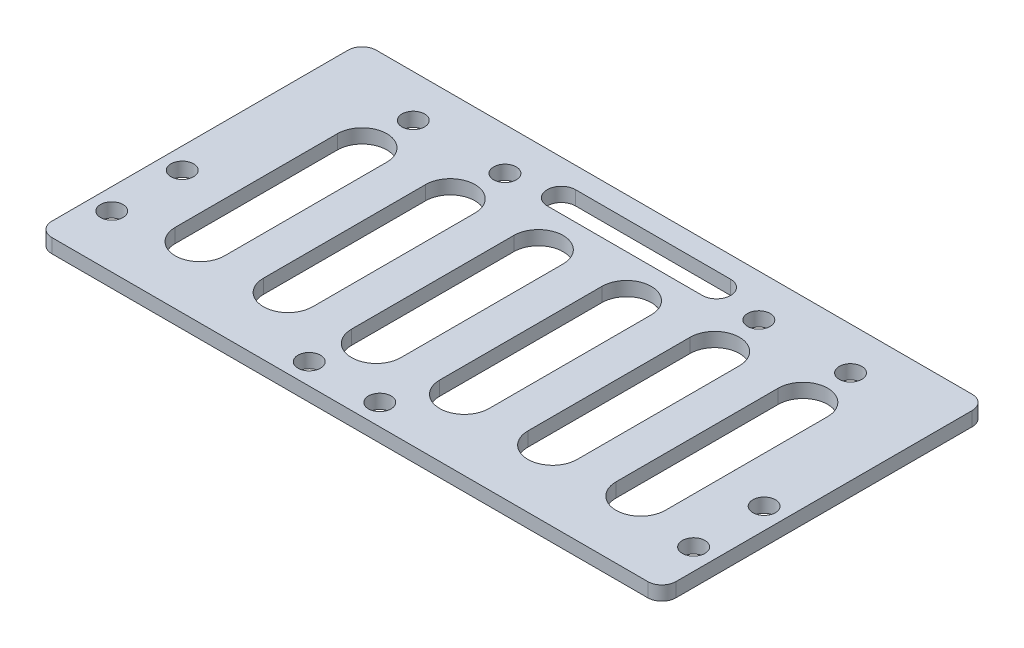
SolidWorks part; units mm, degrees
material "Thornel Mat VMA"
ref_plane "前视基准面" through (0, 0, 0) normal (0, 0, 1) x (1, 0, 0)
ref_plane "上视基准面" through (0, 0, 0) normal (0, 1, 0) x (1, 0, 0)
ref_plane "右视基准面" through (0, 0, 0) normal (1, 0, 0) x (0, 0, -1)
sketch "草图1" plane through (0, 0, 0) normal (0, 1, 0) x (1, 0, 0)
  line L0 (0, 23) -> (0, -23) construction
  line L1 (-44.25, 23) -> (44.25, 23)
  line L2 (-44.25, 23) -> (-44.25, -23)
  line L3 (-44.25, -23) -> (44.25, -23)
  line L4 (44.25, 23) -> (44.25, -23)
  line L5 (-44.25, 23) -> (44.25, -23) construction
  line L6 (-44.25, -23) -> (44.25, 23) construction
  line L7 (-41.25, -5.5) -> (-41.25, -15.5) construction
  line L8 (41.25, -5.5) -> (41.25, -15.5) construction
  line L9 (-8.75, -20) -> (1.25, -20) construction
  line L10 (-31, 17) -> (-18, 17) construction
  line L11 (18, 17) -> (31, 17) construction
  line L12 (-44.25, 0) -> (44.25, 0) construction
  line L13 (-8.75, 20) -> (1.25, 20) construction
  circle A0 centre (-41.25, -5.5) radius 1.6
  circle A1 centre (-41.25, -15.5) radius 1.6
  circle A4 centre (41.25, -15.5) radius 1.6
  circle A5 centre (41.25, -5.5) radius 1.6
  circle A6 centre (-8.75, -20) radius 1.6
  circle A7 centre (1.25, -20) radius 1.6
  circle A8 centre (-31, 17) radius 1.6
  circle A9 centre (-18, 17) radius 1.6
  circle A10 centre (18, 17) radius 1.6
  circle A11 centre (31, 17) radius 1.6
  point P0 (0, 0)
  dimension "D1" = 3.2
  dimension "D7" = 3
  dimension "D9" = 13
  dimension "D11" = 3.2
  dimension "D2" = 3
  dimension "D3" = 7.5
  dimension "D4" = 10
  dimension "D5" = 46
  dimension "D6" = 88.5
  dimension "D8" = 35.5
  dimension "D10" = 6
  dimension "D12" = 36
extrude "凸台-拉伸1" add sketch "草图1" along normal blind 2
sketch "草图2" plane through (0, 2, 0) normal (0, 1, 0) x (1, 0, 0)
  line L0 (0, 23) -> (0, -23) construction
  line L1 (44.25, 23) -> (-44.25, 23) construction
  line L2 (-44.25, -23) -> (44.25, -23) construction
  line L3 (-44.25, -1.5) -> (44.25, -1.5) construction
  line L6 (-31.25, 10) -> (-31.25, -13) construction
  line L7 (-27.75, 10) -> (-27.75, -13)
  line L8 (-34.75, 10) -> (-34.75, -13)
  line L9 (-18.75, 10) -> (-18.75, -13) construction
  line L10 (-15.25, 10) -> (-15.25, -13)
  line L11 (-22.25, 10) -> (-22.25, -13)
  line L12 (-6.25, 10) -> (-6.25, -13) construction
  line L13 (-2.75, 10) -> (-2.75, -13)
  line L14 (-9.75, 10) -> (-9.75, -13)
  line L15 (6.25, 10) -> (6.25, -13) construction
  line L16 (9.75, 10) -> (9.75, -13)
  line L17 (2.75, 10) -> (2.75, -13)
  line L18 (18.75, 10) -> (18.75, -13) construction
  line L19 (22.25, 10) -> (22.25, -13)
  line L20 (15.25, 10) -> (15.25, -13)
  line L21 (31.25, 10) -> (31.25, -13) construction
  line L22 (34.75, 10) -> (34.75, -13)
  line L23 (27.75, 10) -> (27.75, -13)
  line L24 (-44.25, 23) -> (-44.25, -23) construction
  line L27 (44.25, -23) -> (44.25, 23) construction
  line L28 (-11, 18) -> (11, 18) construction
  line L29 (-11, 20) -> (11, 20)
  line L30 (-11, 16) -> (11, 16)
  arc A0 (-27.75, 10) -> (-34.75, 10) centre (-31.25, 10) ccw
  arc A1 (-34.75, -13) -> (-27.75, -13) centre (-31.25, -13) ccw
  arc A2 (-15.25, 10) -> (-22.25, 10) centre (-18.75, 10) ccw
  arc A3 (-22.25, -13) -> (-15.25, -13) centre (-18.75, -13) ccw
  arc A4 (-2.75, 10) -> (-9.75, 10) centre (-6.25, 10) ccw
  arc A5 (-9.75, -13) -> (-2.75, -13) centre (-6.25, -13) ccw
  arc A6 (9.75, 10) -> (2.75, 10) centre (6.25, 10) ccw
  arc A7 (2.75, -13) -> (9.75, -13) centre (6.25, -13) ccw
  arc A8 (22.25, 10) -> (15.25, 10) centre (18.75, 10) ccw
  arc A9 (15.25, -13) -> (22.25, -13) centre (18.75, -13) ccw
  arc A10 (34.75, 10) -> (27.75, 10) centre (31.25, 10) ccw
  arc A11 (27.75, -13) -> (34.75, -13) centre (31.25, -13) ccw
  circle A14 centre (-8.75, -20) radius 1.6 construction
  arc A15 (-11, 20) -> (-11, 16) centre (-11, 18) ccw
  arc A16 (11, 16) -> (11, 20) centre (11, 18) ccw
  point P9 (0, 18)
  point P14 (-31.25, -1.5)
  point P22 (-18.75, -1.5)
  point P29 (-6.25, -1.5)
  point P36 (6.25, -1.5)
  point P43 (18.75, -1.5)
  point P50 (31.25, -1.5)
  dimension "D1" = 3.5
  dimension "D7" = 2
  dimension "D2" = 23
  dimension "D4" = 12.5
  dimension "D5" = 7
  dimension "D6" = 3
  dimension "D8" = 22
  dimension "D3" = 6
extrude "切除-拉伸1" cut sketch "草图2" against normal through all
fillet "圆角1" radius 2 4 edges at (44.25, 1, -23) (44.25, 1, 23) (-44.25, 1, 23) (-44.25, 1, -23)
